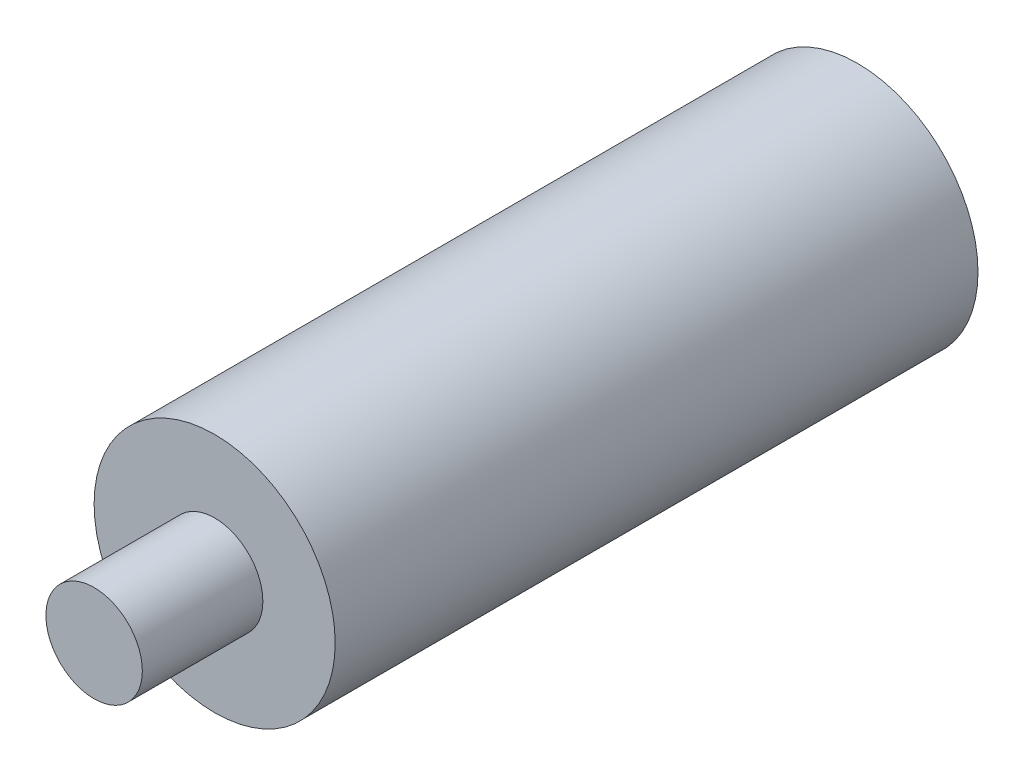
SolidWorks part; units mm, degrees
ref_plane "前视基准面" through (0, 0, 0) normal (0, 0, 1) x (1, 0, 0)
ref_plane "上视基准面" through (0, 0, 0) normal (0, 1, 0) x (1, 0, 0)
ref_plane "右视基准面" through (0, 0, 0) normal (1, 0, 0) x (0, 0, -1)
sketch "草图1" plane through (0, 0, 0) normal (0, 0, 1) x (1, 0, 0)
  circle A0 centre (0, 0) radius 15
  dimension "D1" = 30
extrude "凸台-拉伸1" add sketch "草图1" along normal mid plane 80
hole_wizard "M10 螺纹孔1" positions "草图3" profile "草图2" tap size "M10" standard "GB"
sketch "草图3" plane through (0, 0, -40) normal (0, 0, -1) x (-1, 0, 0)
  circle A0 centre (0, 0) radius 5.5 construction
  point P1 (0, 0)
sketch "草图2" plane through (0, 0, -40) normal (1, 0, 0) x (0, 1, 0)
  line L0 (0, 0) -> (0, 22.5537)
  line L1 (0, 22.5537) -> (4.25, 20)
  line L2 (4.25, 20) -> (4.25, 0)
  line L5 (4.25, 0) -> (0, 0)
  line L10 (0, 22.5537) -> (-4.25, 20) construction
  line L11 (0, -6.35) -> (0, 107.95) construction
  dimension "螺纹孔钻头直径" = 8.5
  dimension "螺纹孔钻头深度" = 20
  dimension "导头角度" = 118
cosmetic thread "孔螺蚊线1" parameters "D1"=20, "D2"=10
sketch "草图4" plane through (0, 0, 40) normal (0, 0, 1) x (1, 0, 0)
  circle A0 centre (0, 0) radius 6
  dimension "D1" = 12
extrude "凸台-拉伸2" add sketch "草图4" along normal blind 15
cosmetic thread "装饰螺纹线1" parameters "D1"=5, "D2"=11
